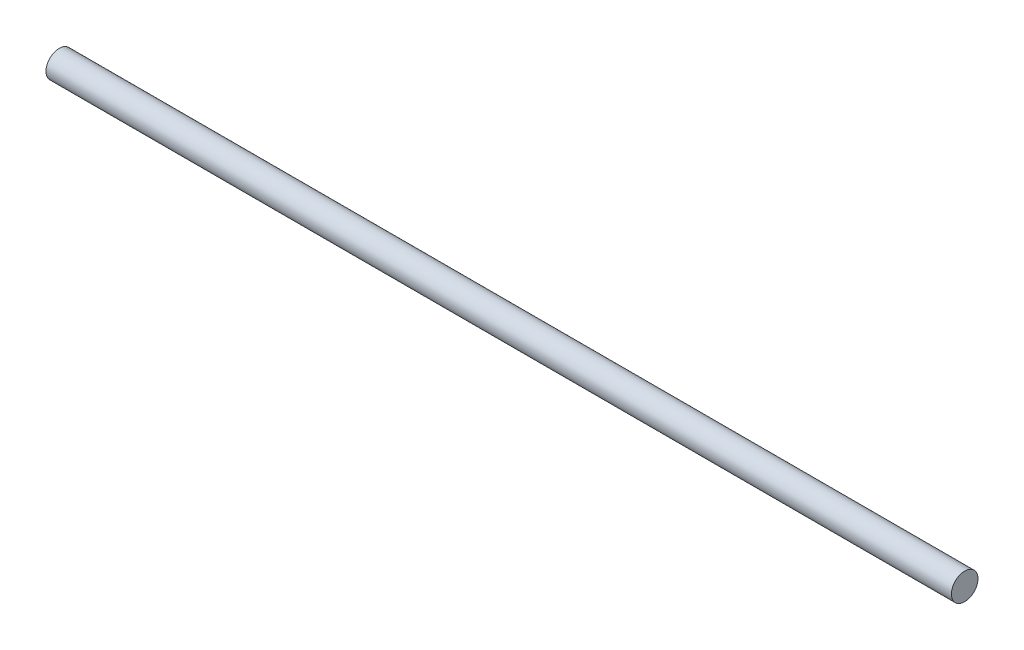
from build123d import *

# Parameters (mm, degrees)
SKETCH12_R          = 15
SKETCH12_R_2        = 12
MEMBER_30X3_1_DEPTH = 1021.5
SKETCH_5_R          = 12
EXTRUDE_2_DEPTH     = 1021.5


with BuildPart() as part:
    # Sketch12 → Member 30X3_1 (new body)
    with BuildSketch(Plane.YZ):
        Circle(SKETCH12_R)
        Circle(SKETCH12_R_2, mode=Mode.SUBTRACT)
    extrude(amount=MEMBER_30X3_1_DEPTH)

    # 草图5 → 凸台-拉伸2 (add, through all)
    with BuildSketch(Plane(origin=(1021.5, 0, 0), x_dir=(0, 0, -1), z_dir=(1, 0, 0))):
        Circle(SKETCH_5_R)
    extrude(amount=-EXTRUDE_2_DEPTH)


solid = part.part
